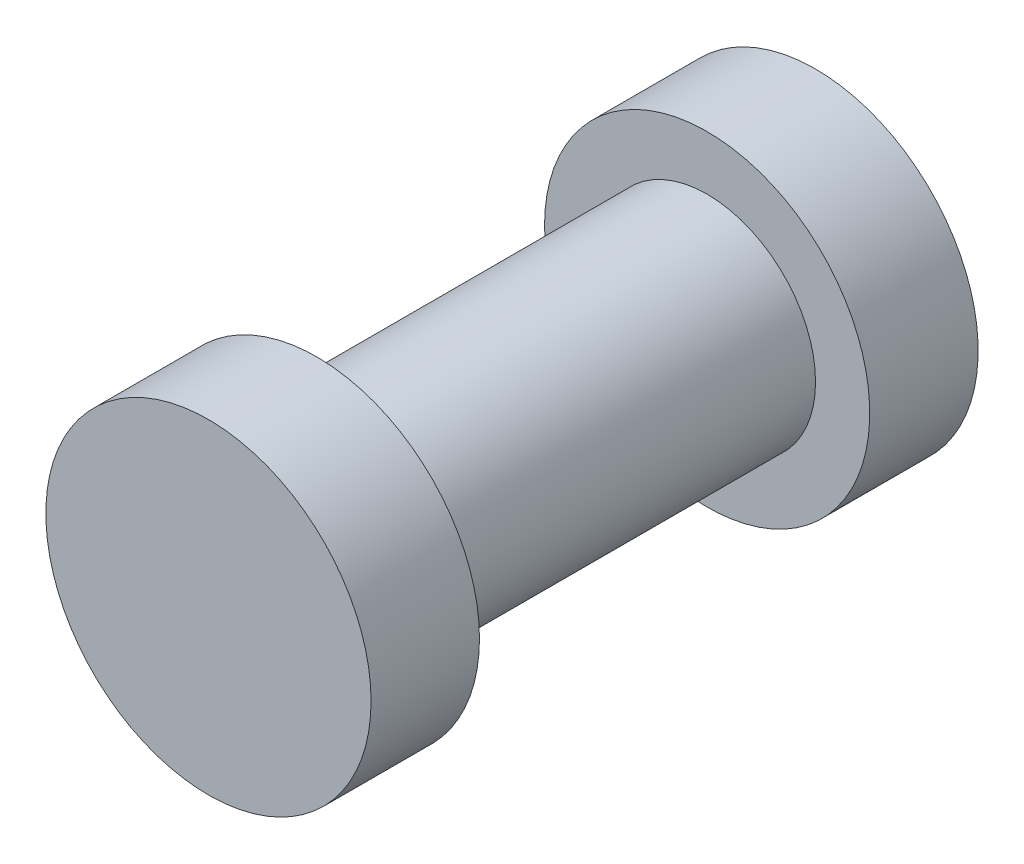
SolidWorks part; units mm, degrees
ref_plane "Front Plane" through (0, 0, 0) normal (0, 0, 1) x (1, 0, 0)
ref_plane "Top Plane" through (0, 0, 0) normal (0, 1, 0) x (1, 0, 0)
ref_plane "Right Plane" through (0, 0, 0) normal (1, 0, 0) x (0, 0, -1)
sketch "Sketch1" plane through (0, 0, 0) normal (0, 0, 1) x (1, 0, 0)
  circle A0 centre (0, 0) radius 10
  dimension "D1" = 20
extrude "Boss-Extrude1" add sketch "Sketch1" along normal blind 36
sketch "Sketch2" plane through (0, 0, 36) normal (0, 0, 1) x (1, 0, 0)
  circle A0 centre (0, 0) radius 15
  dimension "D1" = 30
extrude "Boss-Extrude2" add sketch "Sketch2" along normal blind 10
sketch "Sketch3" plane through (0, 0, 0) normal (0, 0, -1) x (-1, 0, 0)
  circle A0 centre (0, 0) radius 15
  dimension "D1" = 30
extrude "Boss-Extrude3" add sketch "Sketch3" along normal blind 10
